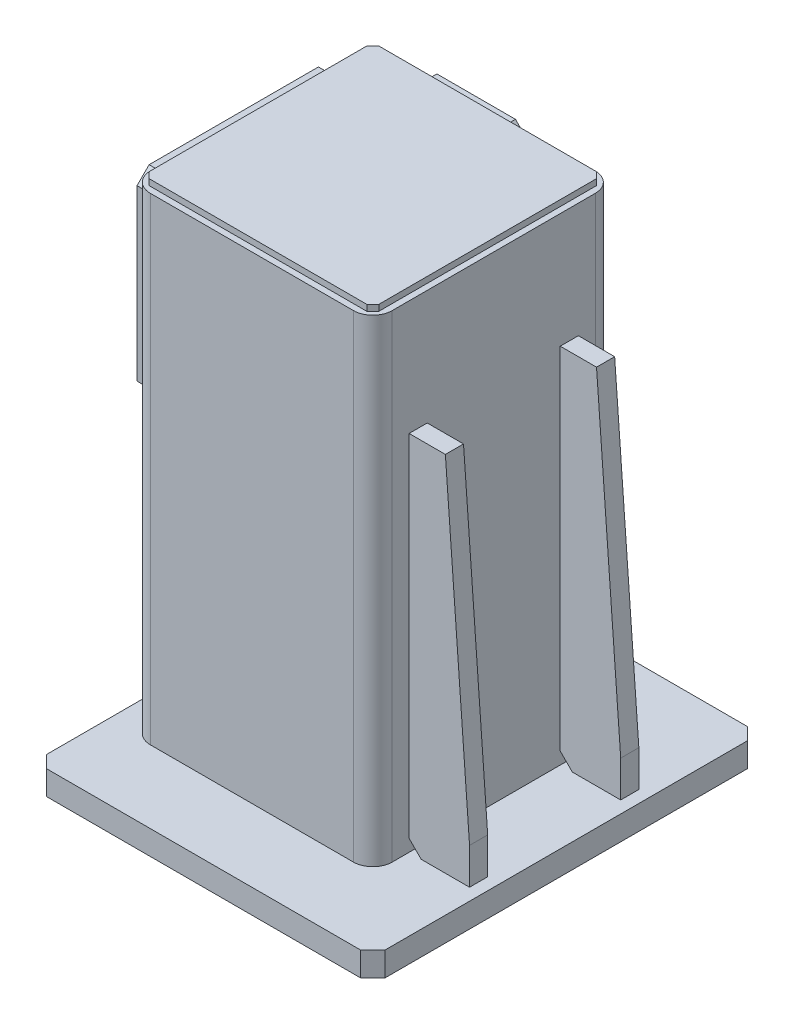
SolidWorks part; units mm, degrees
ref_plane "Front Plane" through (0, 0, 0) normal (0, 0, 1) x (1, 0, 0)
ref_plane "Top Plane" through (0, 0, 0) normal (0, 1, 0) x (1, 0, 0)
ref_plane "Right Plane" through (0, 0, 0) normal (1, 0, 0) x (0, 0, -1)
sketch "Sketch1" plane through (0, 0, 0) normal (0, 1, 0) x (1, 0, 0)
  line L1 (280, 0) -> (280, -320)
  line L6 (280, -160) -> (-66.2364, -160) construction
  line L7 (0, -50) -> (0, -320)
  line L8 (135, -50) -> (0, -50)
  line L9 (135, 0) -> (135, -50)
  line L10 (280, 0) -> (135, 0)
  line L11 (0, -320) -> (280, -320)
  dimension "D1" = 280
  dimension "D2" = 320
  dimension "D3" = 145
  dimension "D4" = 50
  dimension "D5" = 145
extrude "Boss-Extrude1" add sketch "Sketch1" along normal blind 20
sketch "Sketch2" plane through (0, 20, 0) normal (0, 1, 0) x (1, 0, 0)
  line L1 (36, -60) -> (204, -60)
  line L2 (20, -76) -> (20, -244)
  line L3 (36, -260) -> (204, -260)
  line L4 (220, -76) -> (220, -244)
  line L5 (280, -320) -> (280, 0) construction
  line L6 (36, -68) -> (204, -68)
  line L7 (212, -76) -> (212, -244)
  line L8 (36, -252) -> (204, -252)
  line L9 (28, -76) -> (28, -244)
  line L10 (280, 0) -> (135, 0) construction
  arc A0 (204, -260) -> (220, -244) centre (204, -244) ccw
  arc A1 (220, -76) -> (204, -60) centre (204, -76) ccw
  arc A2 (36, -260) -> (20, -244) centre (36, -244) cw
  arc A3 (20, -76) -> (36, -60) centre (36, -76) cw
  arc A4 (212, -76) -> (204, -68) centre (204, -76) ccw
  arc A5 (204, -252) -> (212, -244) centre (204, -244) ccw
  arc A6 (36, -252) -> (28, -244) centre (36, -244) cw
  arc A7 (28, -76) -> (36, -68) centre (36, -76) cw
  dimension "D4" = 16
  dimension "D1" = 200
  dimension "D2" = 60
  dimension "D3" = 60
  dimension "D5" = 8
extrude "Boss-Extrude2" add sketch "Sketch2" along normal blind 395
sketch "Sketch3" plane through (0, 0, 260) normal (0, 0, 1) x (1, 0, 0)
  line L0 (230, 20) -> (270, 20)
  line L1 (270, 20) -> (270, 50)
  line L2 (270, 50) -> (250, 320)
  line L3 (250, 320) -> (220, 320)
  line L4 (220, 415) -> (220, 20) construction
  line L5 (220, 320) -> (220, 30)
  line L6 (220, 30) -> (230, 20)
  point P0 (220, 20)
  dimension "D1" = 30
  dimension "D2" = 30
  dimension "D3" = 300
  dimension "D4" = 50
extrude "Boss-Extrude3" add sketch "Sketch3" against normal blind 15 from offset 30 offset against normal yes
ref_plane "Plane1" through (0, 0, 160) normal (0, 0, -1) x (-1, 0, 0)
mirror "Mirror1" about plane through (0, 0, 160) normal (0, 0, -1) of "Boss-Extrude3"
sketch "Sketch4" plane through (0, 415, 0) normal (0, 1, 0) x (1, 0, 0)
  line L0 (92.4, -160) -> (-92.4, -160) construction
  line L1 (30, -65) -> (210, -65)
  line L2 (25, -70) -> (25, -250)
  line L3 (30, -255) -> (210, -255)
  line L4 (215, -70) -> (215, -250)
  line L5 (20, -76) -> (20, -244) construction
  line L6 (25, -70) -> (30, -65)
  line L7 (25, -250) -> (30, -255)
  line L8 (210, -255) -> (215, -250)
  line L9 (210, -65) -> (215, -70)
  point P0 (25, -65)
  point P1 (215, -255)
  point P2 (25, -255)
  point P3 (215, -65)
  dimension "D1" = 190
  dimension "D2" = 190
  dimension "D3" = 95
  dimension "D4" = 5
extrude "Boss-Extrude4" add sketch "Sketch4" along normal blind 5
sketch "Sketch5" plane through (20, 0, 0) normal (-1, 0, 0) x (0, 0, 1)
  line L0 (160, 380) -> (160, 144.7771) construction
  line L1 (90, 405) -> (230, 405)
  line L2 (80, 395) -> (80, 255)
  line L3 (90, 245) -> (230, 245)
  line L4 (240, 395) -> (240, 255)
  line L5 (60, 415) -> (60, 20) construction
  line L6 (76, 415) -> (244, 415) construction
  line L7 (80, 395) -> (90, 405)
  line L8 (80, 255) -> (90, 245)
  line L9 (230, 245) -> (240, 255)
  line L10 (230, 405) -> (240, 395)
  point P0 (80, 405)
  point P1 (240, 245)
  point P2 (80, 245)
  point P3 (240, 405)
  dimension "D1" = 160
  dimension "D2" = 100
  dimension "D3" = 10
  dimension "D4" = 160
extrude "Boss-Extrude5" add sketch "Sketch5" along normal blind 15
chamfer "Chamfer1" distance 10 angle 45 4 edges at (0, 10, 50) (0, 10, 320) (280, 10, 320) (280, 10, 0)
sketch "Sketch8" plane through (0, 0, 60) normal (0, 0, -1) x (-1, 0, 0)
  line L0 (-118, 399) -> (-53, 399)
  line L1 (-43, 389) -> (-43, 59)
  line L2 (-53, 49) -> (-118, 49)
  line L3 (-128, 59) -> (-128, 389)
  line L4 (-220, 415) -> (-220, 20) construction
  line L5 (-128, 389) -> (-118, 399)
  line L6 (-118, 49) -> (-128, 59)
  line L7 (-43, 59) -> (-53, 49)
  line L8 (-53, 399) -> (-43, 389)
  line L9 (-204, 20) -> (-36, 20) construction
  point P0 (-128, 399)
  point P1 (-43, 399)
  point P3 (-43, 49)
  point P4 (-128, 49)
  dimension "D1" = 92
  dimension "D2" = 85
  dimension "D3" = 29
  dimension "D4" = 350
extrude "Boss-Extrude8" add sketch "Sketch8" along normal blind 20
fillet "Fillet1" radius 5 1 edges at (135, 10, 50)
chamfer "Chamfer2" distance 10 angle 45 1 edges at (135, 10, 0)
